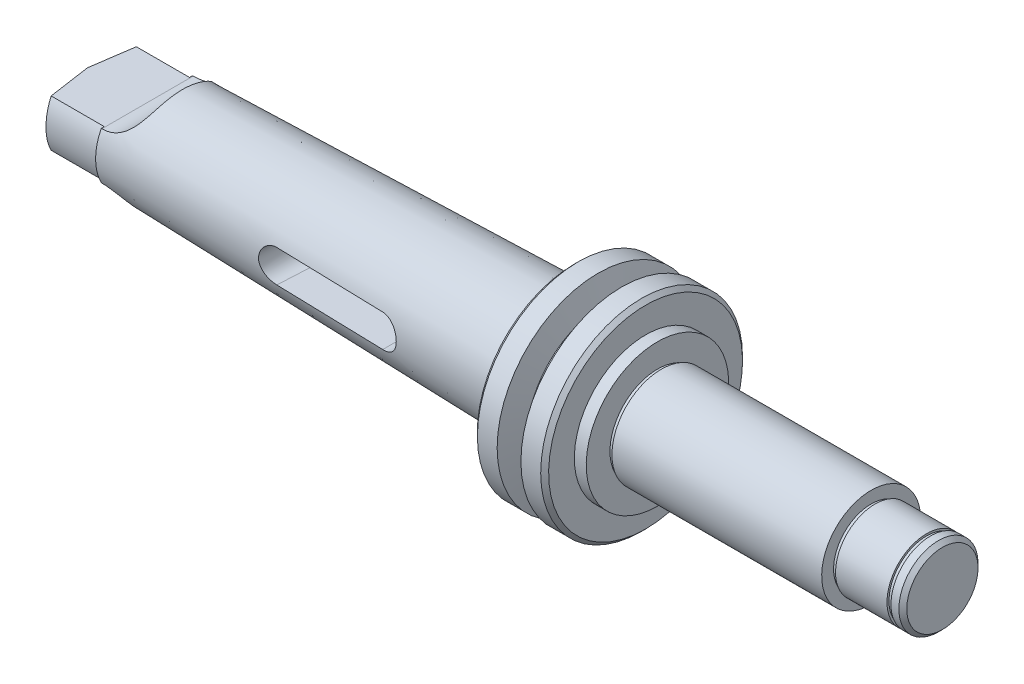
from build123d import *

# Parameters (mm, degrees)
SKETCH7_R               = 12.3
BOSS_EXTRUDE1_DEPTH     = 15
CUT_EXTRUDE5_DEPTH      = 205.209451299
CUT_EXTRUDE5_DEPTH_BACK = 205.209451299
CUT_EXTRUDE6_DEPTH      = 205.209451299
CUT_EXTRUDE6_DEPTH_BACK = 205.209451299
CUT_EXTRUDE7_DEPTH      = 205.209451299
CUT_EXTRUDE7_DEPTH_BACK = 205.209451299
CUT_EXTRUDE8_START      = -6.5
CUT_EXTRUDE8_DEPTH      = 15
CHAMFER1_SIZE           = 1


with BuildPart() as part:
    # Sketch1 → Revolve1 (revolve)
    with BuildSketch(Plane.XY, mode=Mode.PRIVATE) as revolve1_sk:
        Polygon((0, 0), (0, 12.966387971), (108, 15.771), (108, 25.5), (114, 25.5), (115.5, 19.5), (118.5, 19.5), (120, 25.5), (126, 25.5), (126, 18), (129, 18), (129, 12), (130, 12), (130, 12.5), (183, 12.5), (183, 9.5), (184, 9.5), (184, 10), (197, 10), (197, 9.5), (198, 9.5), (198, 10), (201, 10), (201, 0), align=None)
    revolve(revolve1_sk.sketch.rotate(Axis((0, 0, 0), (1, 0, 0)), 180), axis=Axis((0, 0, 0), (1, 0, 0)))

    # Sketch7 → Boss-Extrude1 (add)
    with BuildSketch(Plane.ZY):
        with Locations(Location((0, 0, 0), (0, 0, 270))):
            Circle(SKETCH7_R)
    extrude(amount=BOSS_EXTRUDE1_DEPTH)

    # Sketch8 → Cut-Extrude5 (cut, two sides: drawn at the far end of the back side and taken through both)
    with BuildSketch(Plane.XY.offset(-CUT_EXTRUDE5_DEPTH_BACK)):
        with BuildLine():
            Line((-15, 5.95), (0.171757268, 5.95))
            ThreePointArc((0.171757268, 5.95), (5.883628711, 7.994820303), (9, 13.20010564))
            Line((9, 13.20010564), (-15, 13.20010564))
            Line((-15, 13.20010564), (-15, 5.95))
        make_face()
        with BuildLine():
            Line((-15, -13.20010564), (-15, -5.95))
            Line((-15, -5.95), (0.171757268, -5.95))
            ThreePointArc((0.171757268, -5.95), (5.883628711, -7.994820303), (9, -13.20010564))
            Line((9, -13.20010564), (-15, -13.20010564))
        make_face()
    extrude(amount=CUT_EXTRUDE5_DEPTH + CUT_EXTRUDE5_DEPTH_BACK, mode=Mode.SUBTRACT)

    # Sketch9 → Cut-Extrude6 (cut, two sides: drawn at the far end of the back side and taken through both)
    with BuildSketch(Plane(origin=(0, 0, 0), x_dir=(1, 0, 0), z_dir=(0, 1, 0)).offset(-CUT_EXTRUDE6_DEPTH_BACK)):
        Polygon((-15, 12.3), (-13.205624056, 12.3), (-15, 0), align=None)
        Polygon((-15, -12.3), (-15, 0), (-13.205624056, -12.3), align=None)
    extrude(amount=CUT_EXTRUDE6_DEPTH + CUT_EXTRUDE6_DEPTH_BACK, mode=Mode.SUBTRACT)

    # Sketch10<4> → Cut-Extrude7 (cut, two sides: drawn at the far end of the back side and taken through both)
    with BuildSketch(Plane.XY.offset(-CUT_EXTRUDE7_DEPTH_BACK)):
        with BuildLine():
            Line((47.1, 4.1), (73.9, 4.1))
            ThreePointArc((73.9, 4.1), (78, 0), (73.9, -4.1))
            Line((73.9, -4.1), (47.1, -4.1))
            ThreePointArc((47.1, -4.1), (43, 0), (47.1, 4.1))
        make_face()
    extrude(amount=CUT_EXTRUDE7_DEPTH + CUT_EXTRUDE7_DEPTH_BACK, mode=Mode.SUBTRACT)

    # Cut-Sweep1: sweep along a path in Sketch11
    with BuildLine(Plane(origin=(0, 0, 0), x_dir=(1, 0, 0), z_dir=(0, 1, 0))) as cut_sweep1_path:
        Line((43, 0), (41.163230628, -35.04764745))
    # 草图10<4> → Cut-Sweep1 (sweep, cut)
    with BuildSketch(Plane.XY):
        with BuildLine():
            Line((47.1, 4.1), (73.9, 4.1))
            ThreePointArc((73.9, 4.1), (78, 0), (73.9, -4.1))
            Line((73.9, -4.1), (47.1, -4.1))
            ThreePointArc((47.1, -4.1), (43, 0), (47.1, 4.1))
        make_face()
    cut_sweep1 = sweep(path=cut_sweep1_path.line, mode=Mode.SUBTRACT)

    # Mirror1: Cut-Sweep1 across plane
    add(cut_sweep1.mirror(Plane.XY), mode=Mode.SUBTRACT)

    # Sketch12 → Cut-Extrude8 (cut)
    with BuildSketch(Plane(origin=(0, 0, 0), x_dir=(1, 0, 0), z_dir=(0, 1, 0)).offset(CUT_EXTRUDE8_START)):
        with BuildLine():
            Line((193.5, -3), (187.5, -3))
            ThreePointArc((187.5, -3), (184.5, 0), (187.5, 3))
            Line((187.5, 3), (193.5, 3))
            ThreePointArc((193.5, 3), (196.5, 0), (193.5, -3))
        make_face()
    extrude(amount=-CUT_EXTRUDE8_DEPTH, mode=Mode.SUBTRACT)

    # Chamfer1
    chamfer1_edges = [part.edges().sort_by_distance(p)[0] for p in [
        (201, 10, 0),
        (126, 25.5, 0),
        (108, 25.5, 0),
    ]]
    chamfer(chamfer1_edges, length=CHAMFER1_SIZE)


solid = part.part
